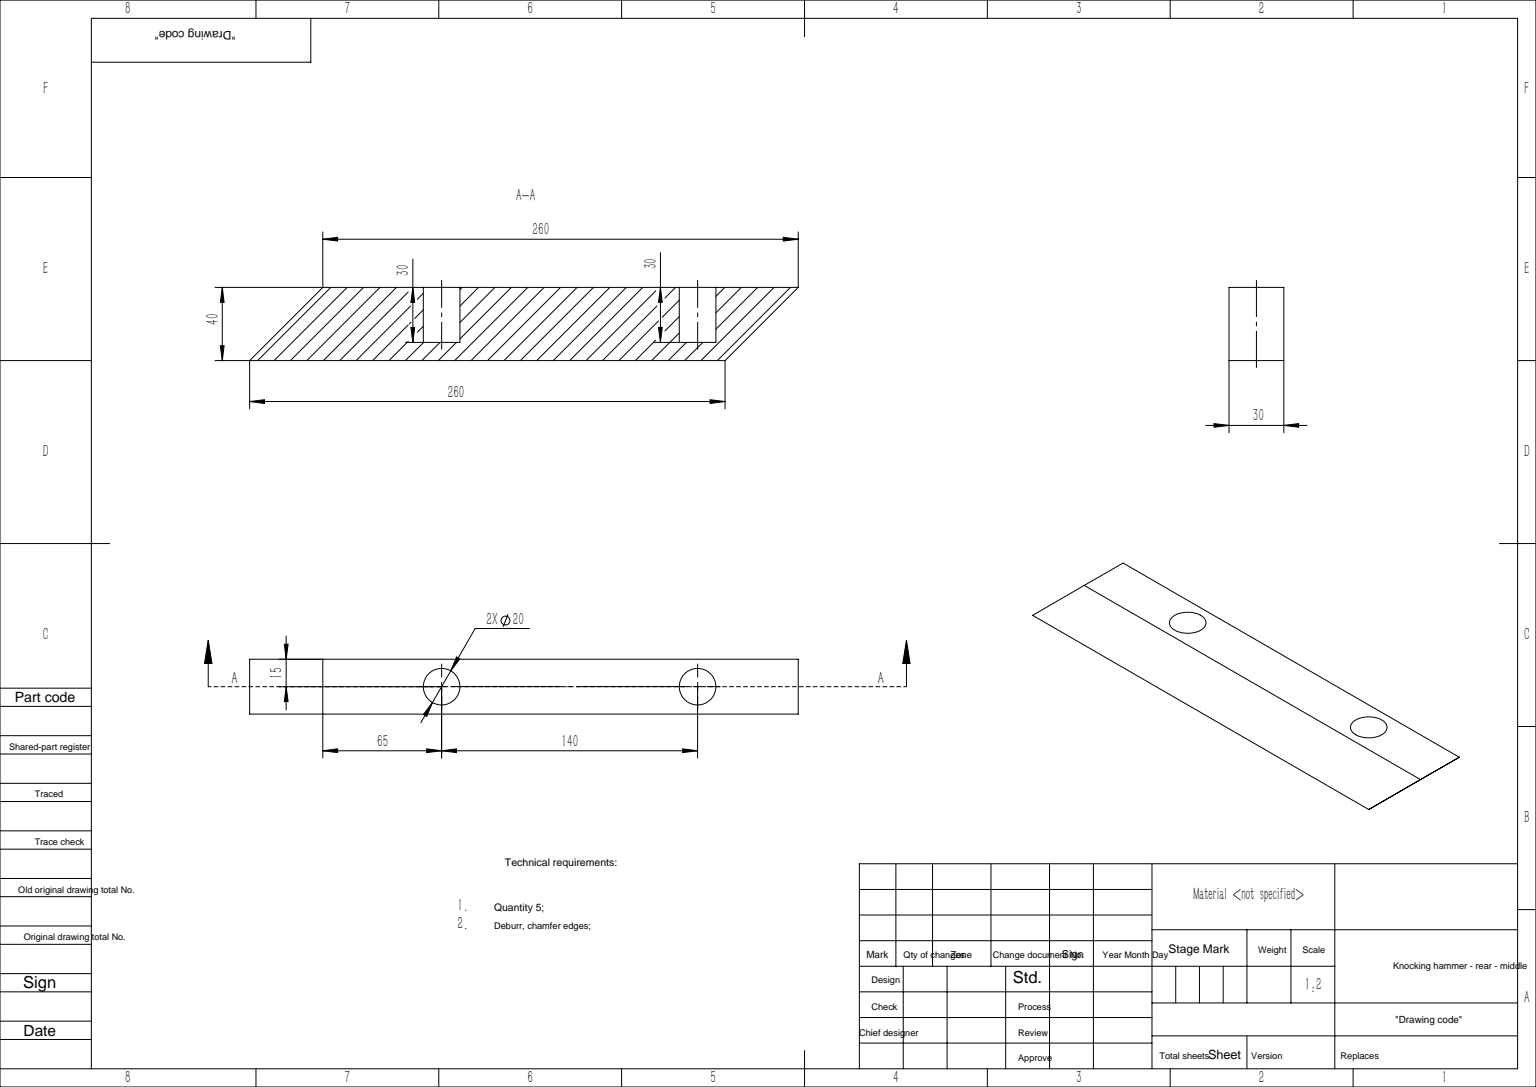
SolidWorks part; units mm, degrees
ref_plane "前视基准面" through (0, 0, 0) normal (0, 0, 1) x (1, 0, 0)
ref_plane "上视基准面" through (0, 0, 0) normal (0, 1, 0) x (1, 0, 0)
ref_plane "右视基准面" through (0, 0, 0) normal (1, 0, 0) x (0, 0, -1)
sketch "草图1" plane through (0, 0, 0) normal (0, 1, 0) x (1, 0, 0)
  line L1 (-135, -15) -> (135, -15)
  line L2 (-135, -15) -> (-135, 15)
  line L3 (-135, 15) -> (135, 15)
  line L4 (135, -15) -> (135, 15)
  line L5 (-135, -15) -> (135, 15) construction
  line L6 (-135, 15) -> (135, -15) construction
  point P0 (0, 0)
  dimension "D1" = 270
  dimension "D2" = 30
extrude "凸台-拉伸1" add sketch "草图1" along normal blind 40
sketch "草图2" plane through (0, 40, 0) normal (0, 1, 0) x (1, 0, 0)
  line L1 (0, 0) -> (0, 40) construction
  circle A0 centre (70, 0) radius 10
  circle A1 centre (-70, 0) radius 10
  dimension "D1" = 20
  dimension "D2" = 140
  dimension "D3" = 40
extrude "切除-拉伸2" cut sketch "草图2" against normal blind 30
sketch "草图7" plane through (135, 0, 0) normal (1, 0, 0) x (0, 0, -1)
  line L4 (-15, 0) -> (15, 0)
  line L5 (15, 0) -> (15, 40)
  line L6 (15, 40) -> (-15, 40)
  line L7 (-15, 40) -> (-15, 0)
  line L8 (-15, 0) -> (15, 0)
  line L9 (15, 0) -> (15, 40)
  line L10 (15, 40) -> (-15, 40)
  line L11 (-15, 40) -> (-15, 0)
  dimension "D1" = 0
extrude "切除-拉伸5" cut sketch "草图7" against normal blind 10
sketch "草图8" plane through (0, 0, 15) normal (0, 0, 1) x (1, 0, 0)
  line L0 (125, 40) -> (85, 0)
  line L1 (-135, 0) -> (125, 0) construction
  line L2 (85, 0) -> (125, 0)
  line L3 (125, 0) -> (125, 40)
  dimension "D1" = 45
extrude "切除-拉伸6" cut sketch "草图8" against normal through all
sketch "草图5" plane through (-135, 0, 0) normal (-1, 0, 0) x (0, 0, 1)
  line L4 (-15, 0) -> (15, 0)
  line L5 (15, 0) -> (15, 40)
  line L6 (15, 40) -> (-15, 40)
  line L7 (-15, 40) -> (-15, 0)
  line L8 (-15, 0) -> (15, 0)
  line L9 (15, 0) -> (15, 40)
  line L10 (15, 40) -> (-15, 40)
  line L11 (-15, 40) -> (-15, 0)
  dimension "D1" = 0
extrude "凸台-拉伸3" add sketch "草图5" along normal blind 40
sketch "草图6" plane through (0, 0, 15) normal (0, 0, 1) x (1, 0, 0)
  line L0 (-175, 0) -> (-135, 40)
  line L1 (-175, 40) -> (125, 40) construction
  line L2 (-135, 40) -> (-175, 40)
  line L3 (-175, 40) -> (-175, 0)
  dimension "D1" = 45
extrude "切除-拉伸4" cut sketch "草图6" against normal through all
